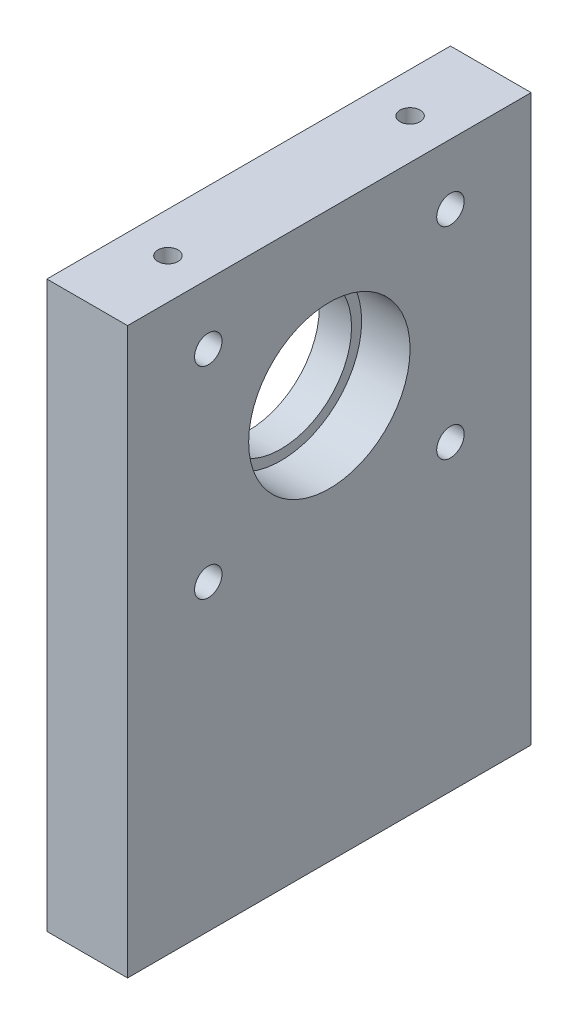
SolidWorks part; units mm, degrees
ref_plane "前视基准面" through (0, 0, 0) normal (0, 0, 1) x (1, 0, 0)
ref_plane "上视基准面" through (0, 0, 0) normal (0, 1, 0) x (1, 0, 0)
ref_plane "右视基准面" through (0, 0, 0) normal (1, 0, 0) x (0, 0, -1)
sketch "草图1" plane through (0, 0, 0) normal (1, 0, 0) x (0, 0, -1)
  line L1 (-50, 70) -> (50, 70)
  line L2 (-50, 70) -> (-50, -70)
  line L3 (-50, -70) -> (50, -70)
  line L4 (50, 70) -> (50, -70)
  line L5 (-50, 70) -> (50, -70) construction
  line L6 (-50, -70) -> (50, 70) construction
  point P0 (0, 0)
  dimension "D1" = 140
  dimension "D2" = 100
extrude "凸台-拉伸1" add sketch "草图1" along normal blind 20
hole_wizard "M10 螺纹孔1" positions "草图2" profile "草图3" tap size "M10" standard "GB"
sketch "草图2" plane through (0, -70, 0) normal (0, -1, 0) x (-1, 0, 0)
  line L0 (-10, 50) -> (-10, -79.2739)
  line L1 (-20, 50) -> (0, 50) construction
  line L3 (0, 0) -> (-46.1818, 0) construction
  point P0 (-10, 30)
  point P2 (-10, -30)
  dimension "D1" = 60
sketch "草图3" plane through (10, -70, -30) normal (1, 0, 0) x (0, 0, -1)
  line L0 (0, 0) -> (0, 27.0537)
  line L1 (0, 27.0537) -> (4.25, 24.5)
  line L2 (4.25, 24.5) -> (4.25, 0)
  line L5 (4.25, 0) -> (0, 0)
  line L10 (0, 27.0537) -> (-4.25, 24.5) construction
  line L11 (0, -6.35) -> (0, 107.95) construction
  dimension "螺纹孔钻头直径" = 8.5
  dimension "螺纹孔钻头深度" = 24.5
  dimension "导头角度" = 118
cosmetic thread "孔螺蚊线1" parameters "D1"=20, "D2"=10
cosmetic thread "孔螺蚊线2" parameters "D1"=20, "D2"=10
sketch "草图4" plane through (20, 0, 0) normal (1, 0, 0) x (0, 0, -1)
  line L0 (-50, -70) -> (50, -70) construction
  circle A0 centre (0, 30) radius 20
  dimension "D2" = 40
  dimension "D1" = 100
extrude "切除-拉伸1" cut sketch "草图4" against normal blind 12
sketch "草图5" plane through (8, 0, 0) normal (1, 0, 0) x (0, 0, -1)
  circle A0 centre (0, 30) radius 17.5
  dimension "D1" = 35
extrude "切除-拉伸2" cut sketch "草图5" against normal through all
hole_wizard "M8 螺纹孔1" positions "草图8" profile "草图9" tap size "M8" standard "GB" end condition through all
sketch "草图8" plane through (0, 0, 0) normal (-1, 0, 0) x (0, 0, 1)
  line L8 (0, 30) -> (30, 30) construction
  point P0 (-30, 55)
  point P18 (30, 55)
  point P20 (-30, 5)
  point P22 (30, 5)
  dimension "D1" = 60
  dimension "D3" = 50
sketch "草图9" plane through (0, 55, -30) normal (0, 1, 0) x (0, 0, 1)
  line L0 (0, 0) -> (0, 20)
  line L1 (0, 20) -> (3.4, 20)
  line L2 (3.4, 20) -> (3.4, 0)
  line L5 (3.4, 0) -> (0, 0)
  line L11 (0, -6.35) -> (0, 107.95) construction
  dimension "通孔螺纹孔钻头直径" = 6.8
  dimension "通孔螺纹孔钻头深度" = 20
cosmetic thread "孔螺蚊线3" parameters "D2"=8
cosmetic thread "孔螺蚊线4" parameters "D2"=8
cosmetic thread "孔螺蚊线5" parameters "D2"=8
cosmetic thread "孔螺蚊线6" parameters "D2"=8
hole_wizard "M6 螺纹孔1" positions "草图10" profile "草图11" tap size "M6" standard "GB"
sketch "草图10" plane through (0, 70, 0) normal (0, 1, 0) x (1, 0, 0)
  line L0 (0, 0) -> (22.1675, 0) construction
  line L2 (10, -50) -> (10, 55.2364) construction
  line L3 (20, -50) -> (0, -50) construction
  point P0 (10, 30)
  point P2 (10, -30)
  dimension "D1" = 60
sketch "草图11" plane through (10, 70, -30) normal (1, 0, 0) x (0, 0, 1)
  line L0 (0, 0) -> (0, 16.5022)
  line L1 (0, 16.5022) -> (2.5, 15)
  line L2 (2.5, 15) -> (2.5, 0)
  line L5 (2.5, 0) -> (0, 0)
  line L10 (0, 16.5022) -> (-2.5, 15) construction
  line L11 (0, -6.35) -> (0, 107.95) construction
  dimension "螺纹孔钻头直径" = 5
  dimension "螺纹孔钻头深度" = 15
  dimension "导头角度" = 118
cosmetic thread "孔螺蚊线7" parameters "D1"=12, "D2"=6
cosmetic thread "孔螺蚊线8" parameters "D1"=12, "D2"=6
